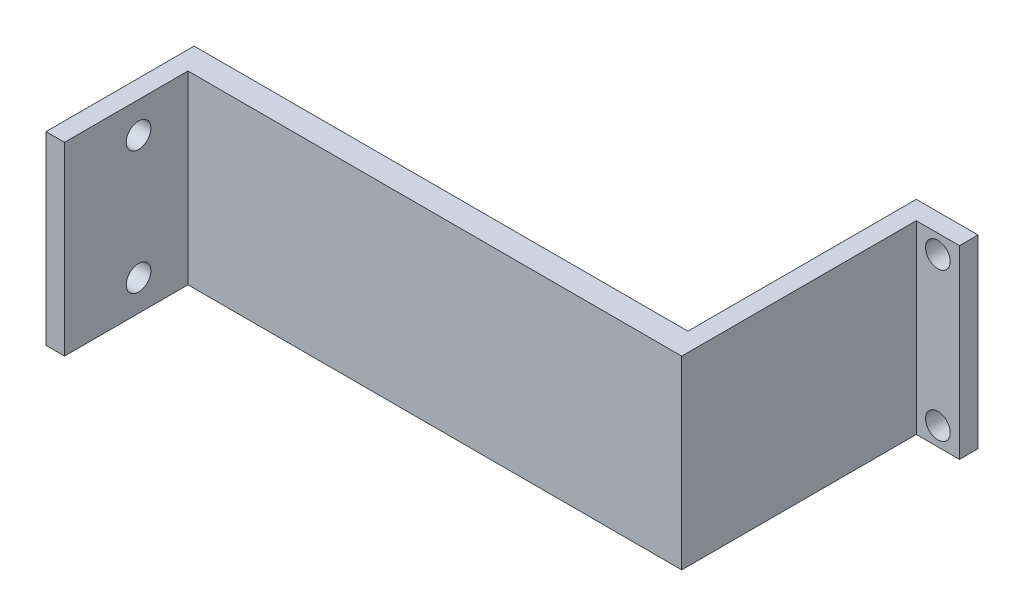
from build123d import *

# Parameters (mm, degrees)
SKETCH_1_W          = 1.5
SKETCH_1_H          = 15
EXTRUDE_1_DEPTH     = 20.5
SKETCH_1_5_W        = 3.5
SKETCH_1_5_H        = 15
EXTRUDE_2_DEPTH     = 1.5
SKETCH_2_R          = 1
CUT_EXTRUDE_1_DEPTH = 1.5
SKETCH_3_W          = 2
SKETCH_3_H          = 15
EXTRUDE_3_DEPTH     = 40
SKETCH_4_W          = 1.5
SKETCH_4_H          = 15
EXTRUDE_4_DEPTH     = 10
SKETCH_5_R          = 1
CUT_EXTRUDE_3_DEPTH = 10


with BuildPart() as part:
    # 草图1 → 凸台-拉伸1 (new body)
    with BuildSketch(Plane.XY):
        with Locations((-1.75, 0)):
            Rectangle(SKETCH_1_W, SKETCH_1_H)
    extrude(amount=EXTRUDE_1_DEPTH)

    # 草图1<5> → 凸台-拉伸2 (add)
    with BuildSketch(Plane.XY):
        with Locations((0.75, 0)):
            Rectangle(SKETCH_1_5_W, SKETCH_1_5_H)
    extrude(amount=EXTRUDE_2_DEPTH)

    # 草图2 → 切除-拉伸1 (cut)
    with BuildSketch(Plane.XY.offset(1.5)):
        with Locations((0.75, 6)):
            Circle(SKETCH_2_R)
        with Locations((0.75, -6)):
            Circle(SKETCH_2_R)
    extrude(amount=-CUT_EXTRUDE_1_DEPTH, mode=Mode.SUBTRACT)

    # 草图3 → 凸台-拉伸3 (add)
    with BuildSketch(Plane.ZY.offset(2.5)):
        with Locations((19.5, 0)):
            Rectangle(SKETCH_3_W, SKETCH_3_H)
    extrude(amount=EXTRUDE_3_DEPTH)

    # 草图4 → 凸台-拉伸4 (add)
    with BuildSketch(Plane.XY.offset(20.5)):
        with Locations((-41.75, 0)):
            Rectangle(SKETCH_4_W, SKETCH_4_H)
    extrude(amount=EXTRUDE_4_DEPTH)

    # 草图5 → 切除-拉伸3 (cut)
    with BuildSketch(Plane.ZY.offset(42.5)):
        with Locations((24.5, 5)):
            Circle(SKETCH_5_R)
        with Locations((24.5, -5)):
            Circle(SKETCH_5_R)
    extrude(amount=-CUT_EXTRUDE_3_DEPTH, mode=Mode.SUBTRACT)


solid = part.part
